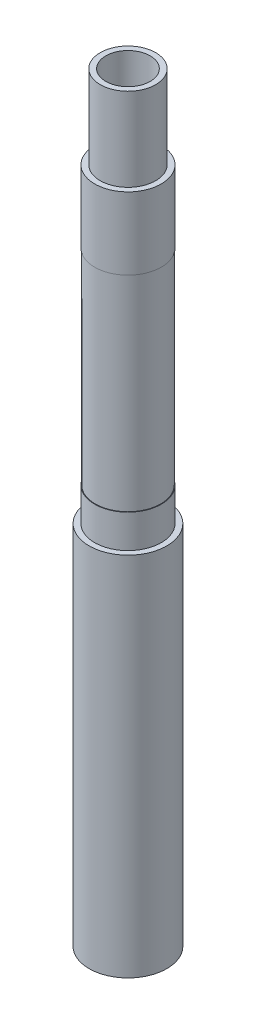
SolidWorks part; units mm, degrees
material "Q235B"
ref_plane "Front Plane" through (0, 0, 0) normal (0, 0, 1) x (1, 0, 0)
ref_plane "Top Plane" through (0, 0, 0) normal (0, 1, 0) x (1, 0, 0)
ref_plane "Right Plane" through (0, 0, 0) normal (1, 0, 0) x (0, 0, -1)
sketch "Sketch1" plane through (0, 0, 0) normal (0, 0, 1) x (1, 0, 0)
  line L0 (0, 0) -> (35, 0)
  line L1 (35, 0) -> (35, 330)
  line L2 (35, 330) -> (30, 330)
  line L3 (30, 330) -> (30, 360)
  line L4 (30, 360) -> (29.5, 360)
  line L5 (29.5, 360) -> (29.5, 545)
  line L6 (29.5, 545) -> (30, 545)
  line L7 (30, 545) -> (30, 610)
  line L8 (30, 610) -> (25, 610)
  line L9 (25, 610) -> (25, 685)
  line L10 (25, 685) -> (0, 685)
  line L11 (0, 685) -> (0, 0) construction
  line L12 (0, 0) -> (0, 685)
  dimension "D1" = 70
  dimension "D2" = 60
  dimension "D3" = 59
  dimension "D4" = 60
  dimension "D5" = 50
  dimension "D6" = 685
  dimension "D7" = 75
  dimension "D8" = 65
  dimension "D9" = 185
  dimension "D10" = 30
revolve "Revolve1" add sketch "Sketch1" angle 360 about L11
cosmetic thread "Cosmetic Thread1" parameters "D1"=35, "D2"=54.046
sketch "Sketch2" plane through (0, 685, 0) normal (0, 1, 0) x (1, 0, 0)
  circle A0 centre (0, 0) radius 20
  dimension "D1" = 40
extrude "Cut-Extrude1" cut sketch "Sketch2" against normal up to next
